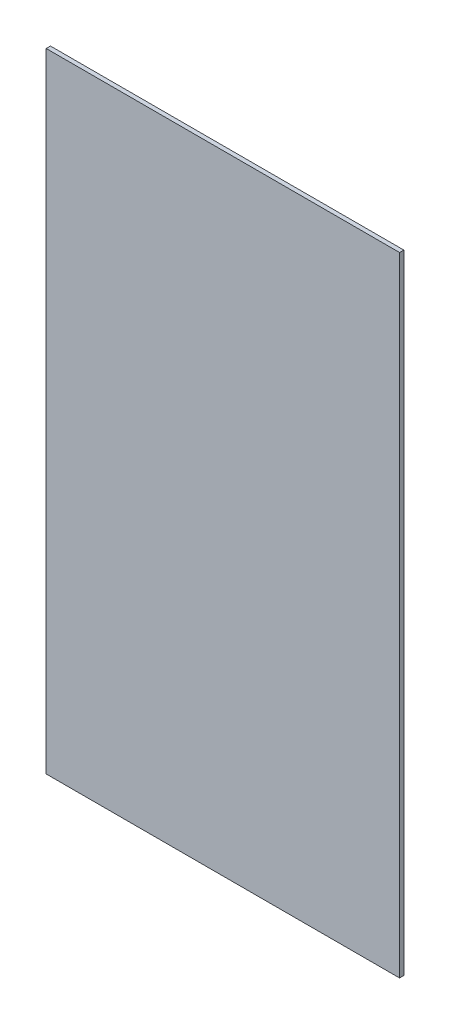
SolidWorks part; units mm, degrees
material "PMMA(有机玻璃)"
ref_plane "前视" through (0, 0, 0) normal (0, 0, 1) x (1, 0, 0)
ref_plane "上视" through (0, 0, 0) normal (0, 1, 0) x (1, 0, 0)
ref_plane "右视" through (0, 0, 0) normal (1, 0, 0) x (0, 0, -1)
sketch "草图1" plane through (0, 0, 0) normal (0, 0, 1) x (1, 0, 0)
  line L1 (-207, 368) -> (207, 368)
  line L2 (-207, 368) -> (-207, -368)
  line L3 (-207, -368) -> (207, -368)
  line L4 (207, 368) -> (207, -368)
  line L5 (-207, 368) -> (207, -368) construction
  line L6 (-207, -368) -> (207, 368) construction
  point P0 (0, 0)
  dimension "D1" = 736
  dimension "D2" = 414
extrude "凸台-拉伸1" add sketch "草图1" along normal blind 5
hole_wizard "M5 间隙孔1" positions "草图3" profile "草图2" hole size "M5" standard "GB"
sketch "草图3" plane through (0, 0, 5) normal (0, 0, 1) x (1, 0, 0)
  line L0 (-427.5, 273) -> (-427.5, -273) construction
  line L1 (-427.5, -273) -> (427.5, -273) construction
  line L2 (0, 273) -> (0, -273) construction
  line L3 (427.5, 273) -> (-427.5, 273) construction
  line L5 (-427.5, 0) -> (427.5, 0) construction
  line L6 (427.5, -273) -> (427.5, 273) construction
  point P0 (-375, -261)
  point P46 (415.5, 250)
  point P48 (-415.5, 250)
  point P58 (-125, -261)
  point P59 (125, -261)
  point P61 (-125, 261)
  point P62 (125, 261)
  point P64 (-375, 261)
  point P88 (375, -261)
  point P89 (375, 261)
  point P108 (415.5, 0)
  point P109 (-415.5, 0)
  point P110 (415.5, -250)
  point P111 (-415.5, -250)
  dimension "D1" = 12
  dimension "D2" = 12
  dimension "D5" = 3
  dimension "D3" = 12
  dimension "D6" = 4
  dimension "D4" = 2
sketch "草图2" plane through (-375, -261, 5) normal (1, 0, 0) x (0, -1, 0)
  line L0 (0, 0) -> (0, 5)
  line L1 (0, 5) -> (2.75, 5)
  line L2 (2.75, 5) -> (2.75, 0)
  line L5 (2.75, 0) -> (0, 0)
  line L11 (0, -6.35) -> (0, 107.95) construction
  dimension "通孔孔直径" = 5.5
  dimension "通孔孔深度" = 5
